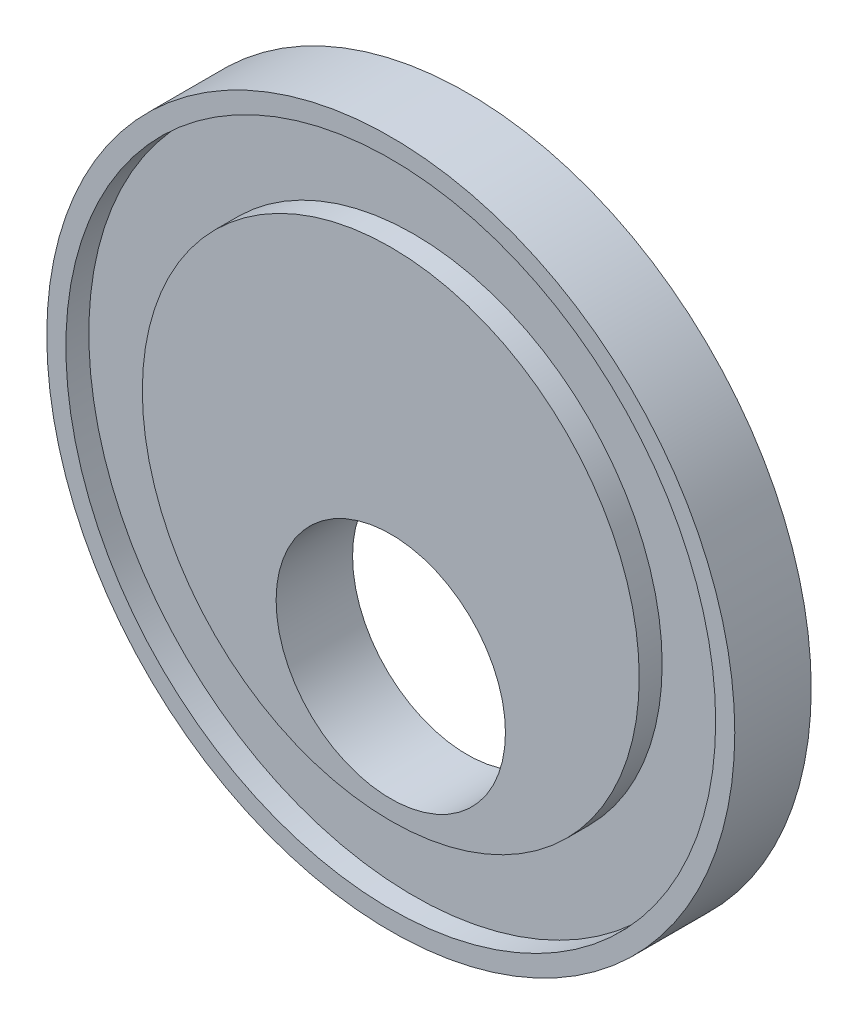
from build123d import *

# Parameters (mm, degrees)
SKETCH1_R           = 90
SKETCH1_R_2         = 30
BOSS_EXTRUDE1_DEPTH = 20
SKETCH2_R           = 85
SKETCH2_R_2         = 65
CUT_EXTRUDE1_DEPTH  = 6
CUT_EXTRUDE2_START  = -6
SKETCH3_R           = 85
SKETCH3_R_2         = 65
CUT_EXTRUDE2_DEPTH  = 6


with BuildPart() as part:
    # Sketch1 → Boss-Extrude1 (new body)
    with BuildSketch(Plane.XY):
        with Locations((0, 30)):
            Circle(SKETCH1_R)
        Circle(SKETCH1_R_2, mode=Mode.SUBTRACT)
    extrude(amount=BOSS_EXTRUDE1_DEPTH)

    # Sketch2 → Cut-Extrude1 (cut)
    with BuildSketch(Plane.XY.offset(20)):
        with Locations((0, 30)):
            Circle(SKETCH2_R)
        with Locations((0, 30)):
            Circle(SKETCH2_R_2, mode=Mode.SUBTRACT)
    extrude(amount=-CUT_EXTRUDE1_DEPTH, mode=Mode.SUBTRACT)

    # Sketch3 → Cut-Extrude2 (cut)
    with BuildSketch(Plane(origin=(0, 0, 0), x_dir=(-1, 0, 0), z_dir=(0, 0, -1)).offset(CUT_EXTRUDE2_START)):
        with Locations(Location((0, 30, 0), (0, 0, 180))):
            Circle(SKETCH3_R)
        with Locations(Location((0, 30, 0), (0, 0, 180))):
            Circle(SKETCH3_R_2, mode=Mode.SUBTRACT)
    extrude(amount=CUT_EXTRUDE2_DEPTH, mode=Mode.SUBTRACT)


solid = part.part
